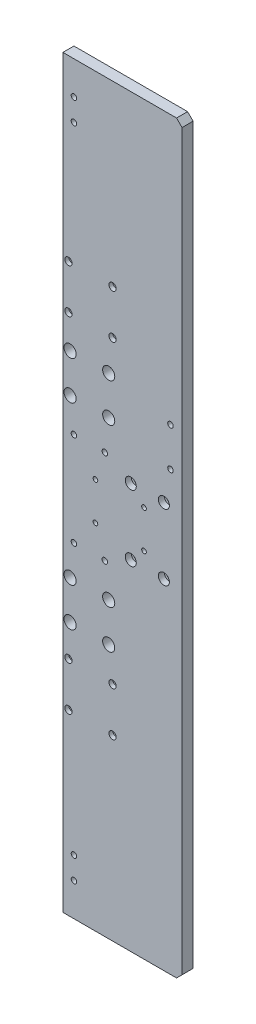
from build123d import *

# Parameters (mm, degrees)
SKETCH_1_W                     = 108
SKETCH_1_H                     = 675
EXTRUDE_1_DEPTH                = 10
HOLE_WIZARD_M6_1_D             = 5
HOLE_WIZARD_M6_1_2_D           = 6.6
HOLE_WIZARD_M6_1_2_CBORE_D     = 11
HOLE_WIZARD_M6_1_2_CBORE_DEPTH = 6.4
HOLE_WIZARD_M5_1_D             = 4.2
HOLE_WIZARD_M5_1_DEPTH         = 14
HOLE_WIZARD_M5_1_TIP           = 1.2618073
HOLE_WIZARD_M6_2_D             = 5
HOLE_WIZARD_M6_2_DEPTH         = 17
HOLE_WIZARD_M6_2_TIP           = 1.502151548
HOLE_WIZARD_M5_1_2_D           = 5.5
HOLE_WIZARD_M5_1_2_DEPTH       = 14
HOLE_WIZARD_M5_1_2_CBORE_D     = 10
HOLE_WIZARD_M5_1_2_CBORE_DEPTH = 5.4
HOLE_WIZARD_M5_1_2_TIP         = 1.652366702
HOLE_WIZARD_M6_3_D             = 5
HOLE_WIZARD_M6_3_DEPTH         = 17
HOLE_WIZARD_M6_3_TIP           = 1.502151548
SKETCH_14_R                    = 5.5
CUT_EXTRUDE_1_DEPTH            = 60
CHAMFER_1_SIZE                 = 5


with BuildPart() as part:
    # 草图1 → 凸台-拉伸1 (new body)
    with BuildSketch(Plane.XY):
        with Locations((54, 337.5)):
            Rectangle(SKETCH_1_W, SKETCH_1_H)
    extrude(amount=EXTRUDE_1_DEPTH)

    # Hole Wizard M6 _1 (through all)
    with Locations(Plane.XY.offset(10)):
        with Locations((10, 645), (10, 625), (10, 50), (10, 30)):
            Hole(HOLE_WIZARD_M6_1_D / 2)

    # Hole Wizard M6 _1 2 (through all)
    with Locations(Plane(origin=(0, 0, 0), x_dir=(-1, 0, 0), z_dir=(0, 0, -1))):
        with Locations((-45, 513.5), (-5, 513.5), (-45, 473.5), (-5, 473.5), (-5, 201.5), (-45, 201.5), (-5, 161.5), (-45, 161.5)):
            CounterBoreHole(HOLE_WIZARD_M6_1_2_D / 2, HOLE_WIZARD_M6_1_2_CBORE_D / 2, HOLE_WIZARD_M6_1_2_CBORE_DEPTH)

    # Hole Wizard M5 _1
    with Locations(Plane.XY.offset(10)):
        with Locations((29.5, 354.5), (73.5, 354.5), (29.5, 320.5), (73.5, 320.5)):
            Hole(HOLE_WIZARD_M5_1_D / 2, depth=HOLE_WIZARD_M5_1_DEPTH)
            with Locations((0, 0, -(HOLE_WIZARD_M5_1_DEPTH + HOLE_WIZARD_M5_1_TIP / 2))):  # 118° drill point
                Cone(0, HOLE_WIZARD_M5_1_D / 2, HOLE_WIZARD_M5_1_TIP, mode=Mode.SUBTRACT)

    # M6 螺纹孔2
    with Locations(Plane.XY.offset(10)):
        with Locations((97.5, 431.5), (97.5, 396.5)):
            Hole(HOLE_WIZARD_M6_2_D / 2, depth=HOLE_WIZARD_M6_2_DEPTH)
            with Locations((0, 0, -(HOLE_WIZARD_M6_2_DEPTH + HOLE_WIZARD_M6_2_TIP / 2))):  # 118° drill point
                Cone(0, HOLE_WIZARD_M6_2_D / 2, HOLE_WIZARD_M6_2_TIP, mode=Mode.SUBTRACT)

    # Hole Wizard M5 _1 2
    with Locations(Plane.XY.offset(10)):
        with Locations((61.5, 367.5), (91.5, 367.5), (61.5, 307.5), (91.5, 307.5)):
            CounterBoreHole(HOLE_WIZARD_M5_1_2_D / 2, HOLE_WIZARD_M5_1_2_CBORE_D / 2, HOLE_WIZARD_M5_1_2_CBORE_DEPTH, depth=HOLE_WIZARD_M5_1_2_DEPTH)
            with Locations((0, 0, -(HOLE_WIZARD_M5_1_2_DEPTH + HOLE_WIZARD_M5_1_2_TIP / 2))):  # 118° drill point
                Cone(0, HOLE_WIZARD_M5_1_2_D / 2, HOLE_WIZARD_M5_1_2_TIP, mode=Mode.SUBTRACT)

    # M6 螺纹孔3
    with Locations(Plane(origin=(0, 0, 0), x_dir=(-1, 0, 0), z_dir=(0, 0, -1))):
        with Locations((-38, 380), (-10, 380), (-38, 295), (-10, 295)):
            Hole(HOLE_WIZARD_M6_3_D / 2, depth=HOLE_WIZARD_M6_3_DEPTH)
            with Locations((0, 0, -(HOLE_WIZARD_M6_3_DEPTH + HOLE_WIZARD_M6_3_TIP / 2))):  # 118° drill point
                Cone(0, HOLE_WIZARD_M6_3_D / 2, HOLE_WIZARD_M6_3_TIP, mode=Mode.SUBTRACT)

    # 草图14 → 切除-拉伸1 (cut)
    with BuildSketch(Plane.XY.offset(10)):
        with Locations((41.5, 444)):
            Circle(SKETCH_14_R)
        with Locations((6.5, 444)):
            Circle(SKETCH_14_R)
        with Locations((41.5, 409)):
            Circle(SKETCH_14_R)
        with Locations((6.5, 409)):
            Circle(SKETCH_14_R)
        with Locations((41.5, 266)):
            Circle(SKETCH_14_R)
        with Locations((41.5, 231)):
            Circle(SKETCH_14_R)
        with Locations((6.5, 231)):
            Circle(SKETCH_14_R)
        with Locations((6.5, 266)):
            Circle(SKETCH_14_R)
    extrude(amount=-CUT_EXTRUDE_1_DEPTH, mode=Mode.SUBTRACT)

    # 倒角1
    chamfer_1_edges = [part.edges().sort_by_distance(p)[0] for p in [
        (108, 0, 5),
        (108, 675, 5),
    ]]
    chamfer(chamfer_1_edges, length=CHAMFER_1_SIZE)


solid = part.part
